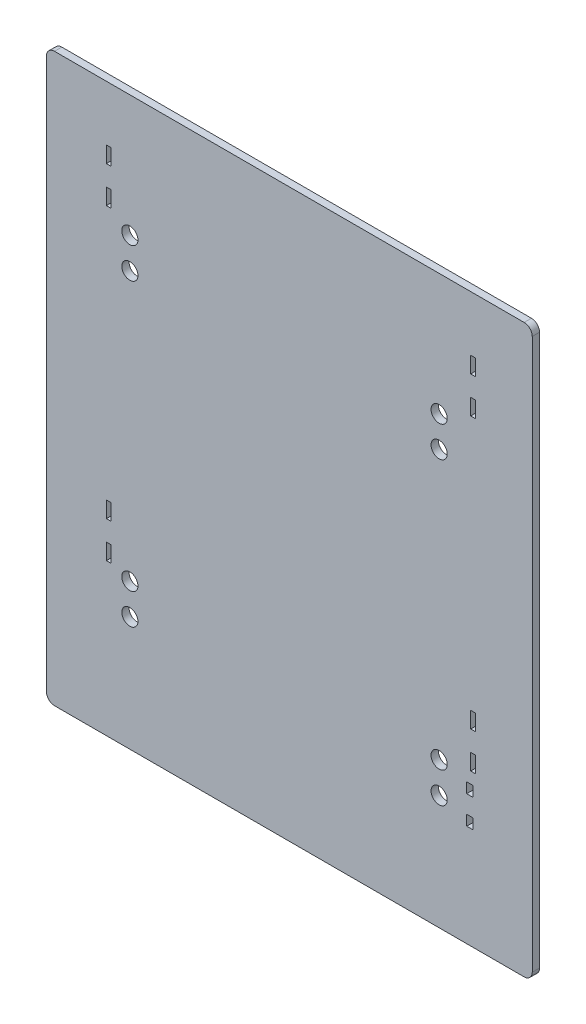
SolidWorks part; units mm, degrees
ref_plane "Front Plane" through (0, 0, 0) normal (0, 0, 1) x (1, 0, 0)
ref_plane "Top Plane" through (0, 0, 0) normal (0, 1, 0) x (1, 0, 0)
ref_plane "Right Plane" through (0, 0, 0) normal (1, 0, 0) x (0, 0, -1)
sketch "Sketch1" plane through (0, 0, 0) normal (0, 0, 1) x (1, 0, 0)
  line L1 (-300, 350) -> (300, 350)
  line L2 (-300, 350) -> (-300, -350)
  line L3 (-300, -350) -> (300, -350)
  line L4 (300, 350) -> (300, -350)
  line L5 (-300, 350) -> (300, -350) construction
  line L6 (-300, -350) -> (300, 350) construction
  point P0 (0, 0)
  dimension "D1" = 600
  dimension "D2" = 700
extrude "Boss-Extrude1" add sketch "Sketch1" along normal blind 9
fillet "Fillet1" radius 10 4 edges at (300, -350, 4.5) (-300, -350, 4.5) (-300, 350, 4.5) (300, 350, 4.5)
extrude "Cut-Extrude2" cut sketch "Sketch3" against normal blind 41
sketch "Sketch3" plane through (-23.018, 7.9334, 0) normal (0, 0, -1) x (-1, 0, 0)
  circle A0 centre (-208.018, 153.6666) radius 10
  circle A1 centre (-208.018, -216.3334) radius 10
  circle A2 centre (-208.018, -178.2334) radius 10
  circle A3 centre (173.982, 191.7666) radius 10
  circle A4 centre (173.982, 153.6666) radius 10
  circle A5 centre (173.982, -178.2334) radius 10
  circle A6 centre (173.982, -216.3334) radius 10
  circle A7 centre (-208.018, 191.7666) radius 10
extrude "Cut-Extrude4" cut sketch "Sketch7" against normal through all
sketch "Sketch7" plane through (-23.018, 7.9334, 0) normal (0, 0, -1) x (-1, 0, 0)
  line L8 (-242.018, -197.4797) -> (-242.018, -184.7319)
  line L10 (-250.018, -184.7319) -> (-250.018, -197.4797)
  line L11 (-250.018, -197.4797) -> (-242.018, -197.4797)
  line L12 (-242.018, -232.2274) -> (-242.018, -219.4797)
  line L13 (-242.018, -219.4797) -> (-250.018, -219.4797)
  line L14 (-250.018, -219.4797) -> (-250.018, -232.2274)
  line L16 (-250.018, -232.2274) -> (-242.018, -232.2274)
  line L17 (-250.018, -184.7319) -> (-242.018, -184.7319)
extrude "Cut-Extrude8" cut sketch "Sketch11" against normal through all both and the other way through all from surface at -116.4038 starting at face at (223, -183.1724, 0)
sketch "Sketch11" plane through (-23.018, 7.9304, -116.4044) normal (0, -0.0001, -1) x (-1, 0, 0)
  line L8 (196.982, -105.8003) -> (196.982, -125.7899)
  line L9 (196.982, -125.7899) -> (202.982, -125.7899)
  line L10 (202.982, -125.7899) -> (202.982, -105.8003)
  line L11 (202.982, -105.8003) -> (196.982, -105.8003)
  line L12 (196.982, -150.8067) -> (196.982, -170.7343)
  line L13 (196.982, -170.7343) -> (202.982, -170.7343)
  line L14 (202.982, -170.7343) -> (202.982, -150.8067)
  line L15 (202.982, -150.8067) -> (196.982, -150.8067)
pattern_linear "LPattern4" count 2 spacing 379.75 along (0, 1, -0.0001) of "Cut-Extrude8"
pattern_linear "LPattern5" count 2 spacing 450 along (1, 0, 0) of "LPattern4", "Cut-Extrude8"
